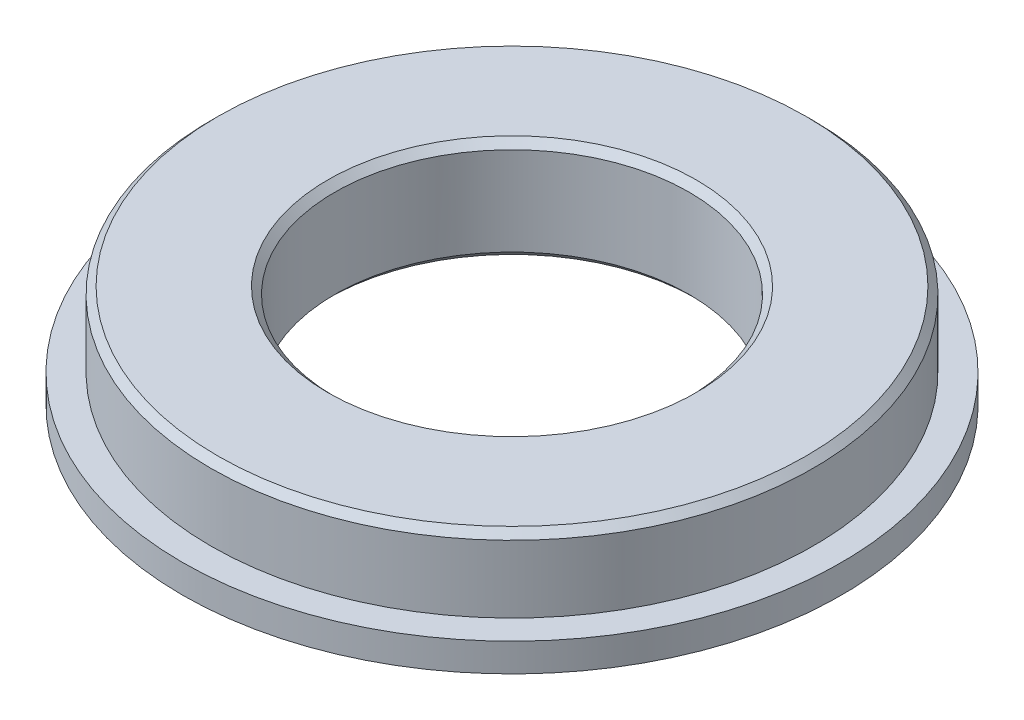
from build123d import *

# Parameters (mm, degrees)
M4_TAPPED_HOLE1_D     = 3.3
M4_TAPPED_HOLE1_DEPTH = 9.8
M4_TAPPED_HOLE1_TIP   = 0.991420021
CHAMFER1_SIZE         = 1


with BuildPart() as part:
    # Sketch1 → Revolve1 (revolve)
    with BuildSketch(Plane.XY, mode=Mode.PRIVATE) as revolve1_sk:
        Polygon((25, 0), (46.5, 0), (46.5, 4), (42.5, 4), (42.5, 14.5), (25, 14.5), align=None)
    revolve(revolve1_sk.sketch.rotate(Axis((0, 0, 0), (0, 1, 0)), 90), axis=Axis((0, 0, 0), (0, 1, 0)))

    # M4 Tapped Hole1
    with Locations(Plane(origin=(0, 0, 0), x_dir=(-1, 0, 0), z_dir=(0, -1, 0))):
        with Locations((0, -36.5), (-31.609927238, -18.25), (-31.609927238, 18.25), (0, 36.5), (31.609927238, 18.25), (31.609927238, -18.25)):
            Hole(M4_TAPPED_HOLE1_D / 2, depth=M4_TAPPED_HOLE1_DEPTH)
            with Locations((0, 0, -(M4_TAPPED_HOLE1_DEPTH + M4_TAPPED_HOLE1_TIP / 2))):  # 118° drill point
                Cone(0, M4_TAPPED_HOLE1_D / 2, M4_TAPPED_HOLE1_TIP, mode=Mode.SUBTRACT)

    # Chamfer1
    chamfer1_edges = [part.edges().sort_by_distance(p)[0] for p in [
        (0, 0, 25),
        (0, 14.5, 25),
        (0, 14.5, 42.5),
    ]]
    chamfer(chamfer1_edges, length=CHAMFER1_SIZE)


solid = part.part
